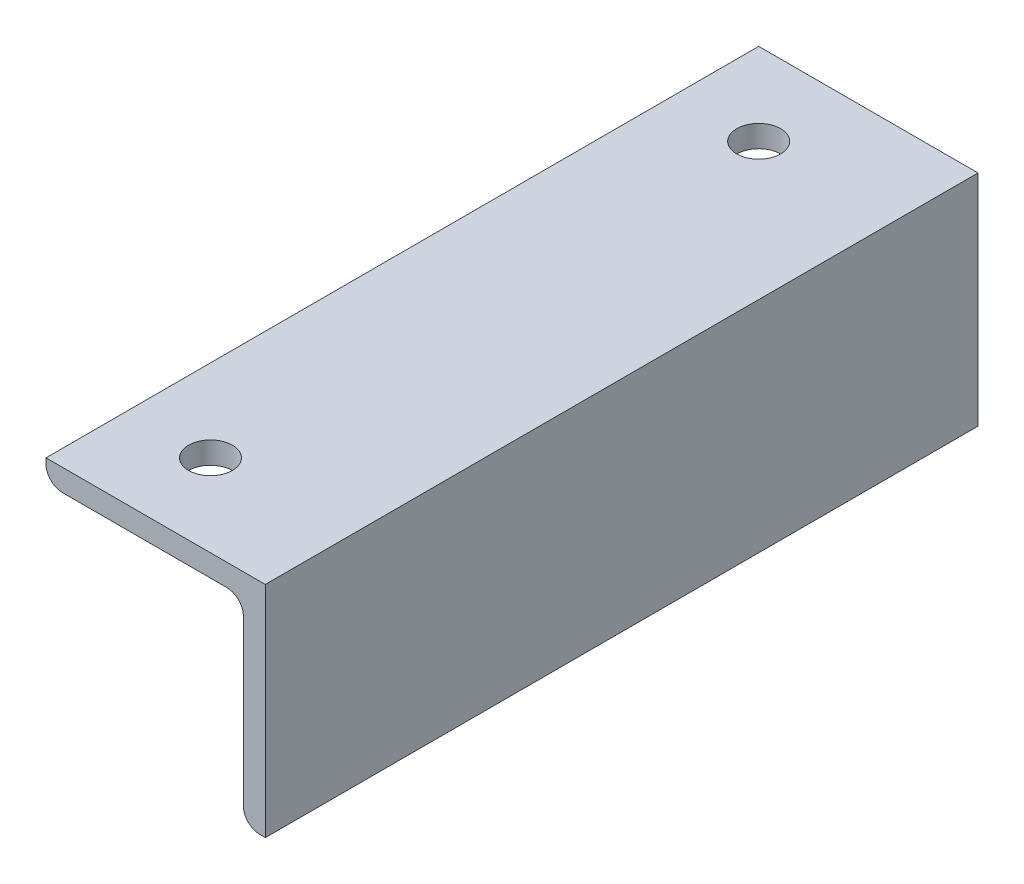
SolidWorks part; units mm, degrees
material "1023 Carbon Steel Plate (SS)"
ref_plane "Front Plane" through (0, 0, 0) normal (0, 0, 1) x (1, 0, 0)
ref_plane "Top Plane" through (0, 0, 0) normal (0, 1, 0) x (1, 0, 0)
ref_plane "Right Plane" through (0, 0, 0) normal (1, 0, 0) x (0, 0, -1)
sketch "Sketch1" plane through (0, 0, 0) normal (0, 0, 1) x (1, 0, 0)
  line L0 (0, 0) -> (40, 0)
  line L1 (40, 0) -> (40, -40)
  line L2 (0, -4) -> (36, -4)
  line L3 (36, -4) -> (36, -40)
  line L4 (0, 0) -> (0, -4)
  line L5 (40, -40) -> (36, -40)
  dimension "D1" = 40
  dimension "D2" = 40
  dimension "D3" = 4
extrude "Boss-Extrude1" add sketch "Sketch1" along normal blind 130 contours L5 L3 L2 L4 L0 L1
fillet "Fillet1" radius 3 3 edges at (36, -4, 65) (36, -40, 65) (0, -4, 65)
sketch "Sketch2" plane through (0, -4, 0) normal (0, -1, 0) x (1, 0, 0)
  line L0 (39, 130) -> (39, 0) construction
  line L1 (40, 130) -> (40, 0) construction
  circle A0 centre (15, 115) radius 4
  circle A1 centre (15, 15) radius 4
  point P6 (39, 65)
  dimension "D2" = 50
  dimension "D4" = 8
  dimension "D1" = 100
  dimension "D3" = 25
extrude "Cut-Extrude1" cut sketch "Sketch2" against normal blind 130
